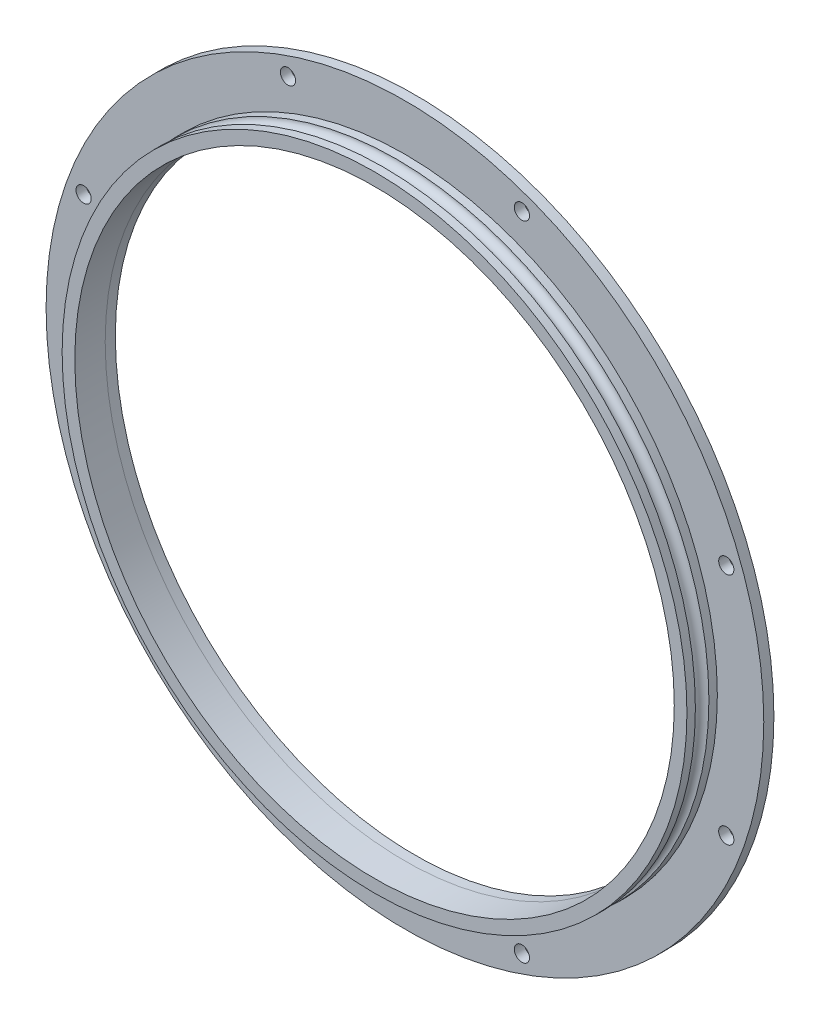
SolidWorks part; units mm, degrees
ref_plane "前视基准面" through (0, 0, 0) normal (0, 0, 1) x (1, 0, 0)
ref_plane "上视基准面" through (0, 0, 0) normal (0, 1, 0) x (1, 0, 0)
ref_plane "右视基准面" through (0, 0, 0) normal (1, 0, 0) x (0, 0, -1)
sketch "草图1" plane through (0, 0, 0) normal (0, 0, 1) x (1, 0, 0)
  circle A0 centre (0, 0) radius 425
  circle A1 centre (0, 0) radius 355
  circle A2 centre (0, 0) radius 410 construction
  dimension "D1" = 850
  dimension "D3" = 15
  dimension "D2" = 70
extrude "凸台-拉伸1" add sketch "草图1" along normal blind 12
sketch "草图2" plane through (0, 0, 12) normal (0, 0, 1) x (1, 0, 0)
  circle A0 centre (0, 0) radius 355
  circle A1 centre (0, 0) radius 370
  dimension "D1" = 15
extrude "凸台-拉伸2" add sketch "草图2" along normal blind 36 separate body
ref_plane "基准面1" through (0, 0, 30) normal (0, 0, -1) x (-1, 0, 0)
sketch "草图3" plane through (0, 0, 30) normal (0, 0, -1) x (-1, 0, 0)
  circle A0 centre (0, 0) radius 370
  circle A1 centre (0, 0) radius 370 construction
sweep "切除-扫描1" cut path "草图3" circular profile diameter 16 parameters "D3"=16
sketch "草图12" plane through (0, 0, 12) normal (0, 0, 1) x (1, 0, 0)
  line L0 (0, 0) -> (240.9699, 0) construction
  line L1 (0, 0) -> (0, 214.6404) construction
  circle A0 centre (0, 0) radius 405 construction
  circle A1 centre (-138.5, 380.5821) radius 9
  circle A2 centre (138.5, 380.5821) radius 9
  circle A3 centre (138.5, -380.5821) radius 9
  circle A4 centre (-138.5, -380.5821) radius 9
  circle A5 centre (-380.5821, 138.5) radius 9
  circle A6 centre (-380.5821, -138.5) radius 9
  circle A7 centre (380.5821, -138.5) radius 9
  circle A8 centre (380.5821, 138.5) radius 9
  point P16 (0, 0)
  dimension "D1" = 810
  dimension "D3" = 18
  dimension "D6" = 761.1642
  dimension "D2" = 277
  dimension "D4" = 138.5
  dimension "D5" = 277
extrude "切除-拉伸1" cut sketch "草图12" against normal blind 20
